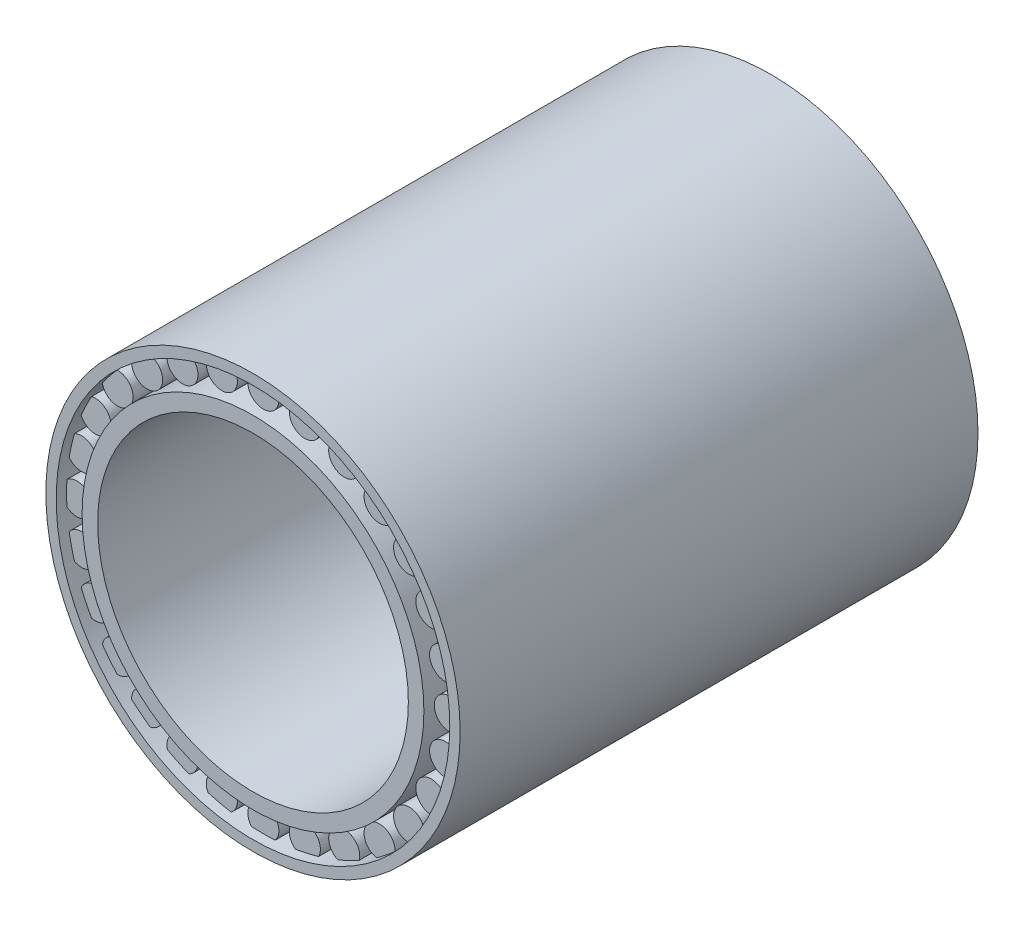
SolidWorks part; units mm, degrees
ref_plane "Front Plane" through (0, 0, 0) normal (0, 0, 1) x (1, 0, 0)
ref_plane "Top Plane" through (0, 0, 0) normal (0, 1, 0) x (1, 0, 0)
ref_plane "Right Plane" through (0, 0, 0) normal (1, 0, 0) x (0, 0, -1)
other "Configuration Table"
sketch "Sketch1" plane through (0, 0, 0) normal (0, 0, 1) x (1, 0, 0)
  circle A0 centre (0, 0) radius 15
  circle A1 centre (0, 0) radius 16.5
  dimension "D1" = 30
  dimension "D2" = 33
extrude "Boss-Extrude1" add sketch "Sketch1" along normal blind 50
sketch "Sketch2" plane through (0, 0, 50) normal (0, 0, 1) x (1, 0, 0)
  circle A0 centre (0, 18) radius 1.5
  circle A1 centre (4.0054, 17.5487) radius 1.5
  circle A2 centre (7.8099, 16.2174) radius 1.5
  circle A3 centre (11.2228, 14.073) radius 1.5
  circle A4 centre (14.073, 11.2228) radius 1.5
  circle A5 centre (16.2174, 7.8099) radius 1.5
  circle A6 centre (17.5487, 4.0054) radius 1.5
  circle A7 centre (18, 0) radius 1.5
  circle A8 centre (17.5487, -4.0054) radius 1.5
  circle A9 centre (16.2174, -7.8099) radius 1.5
  circle A10 centre (14.073, -11.2228) radius 1.5
  circle A11 centre (11.2228, -14.073) radius 1.5
  circle A12 centre (7.8099, -16.2174) radius 1.5
  circle A13 centre (4.0054, -17.5487) radius 1.5
  circle A14 centre (0, -18) radius 1.5
  circle A15 centre (-4.0054, -17.5487) radius 1.5
  circle A16 centre (-7.8099, -16.2174) radius 1.5
  circle A17 centre (-11.2228, -14.073) radius 1.5
  circle A18 centre (-14.073, -11.2228) radius 1.5
  circle A19 centre (-16.2174, -7.8099) radius 1.5
  circle A20 centre (-17.5487, -4.0054) radius 1.5
  circle A21 centre (-18, 0) radius 1.5
  circle A22 centre (-17.5487, 4.0054) radius 1.5
  circle A23 centre (-16.2174, 7.8099) radius 1.5
  circle A24 centre (-14.073, 11.2228) radius 1.5
  circle A25 centre (-11.2228, 14.073) radius 1.5
  circle A26 centre (-7.8099, 16.2174) radius 1.5
  circle A27 centre (-4.0054, 17.5487) radius 1.5
  point P59 (0, 0)
  dimension "D1" = 3
  dimension "D2" = 18
  dimension "D3" = 28
extrude "Boss-Extrude2" add sketch "Sketch2" against normal blind 48 from offset 1 separate body offset against normal yes
sketch "Sketch3" plane through (0, 0, 50) normal (0, 0, 1) x (1, 0, 0)
  circle A0 centre (0, 0) radius 20
  circle A1 centre (0, 0) radius 19
  dimension "D1" = 40
  dimension "D2" = 38
extrude "Boss-Extrude3" add sketch "Sketch3" against normal blind 50
